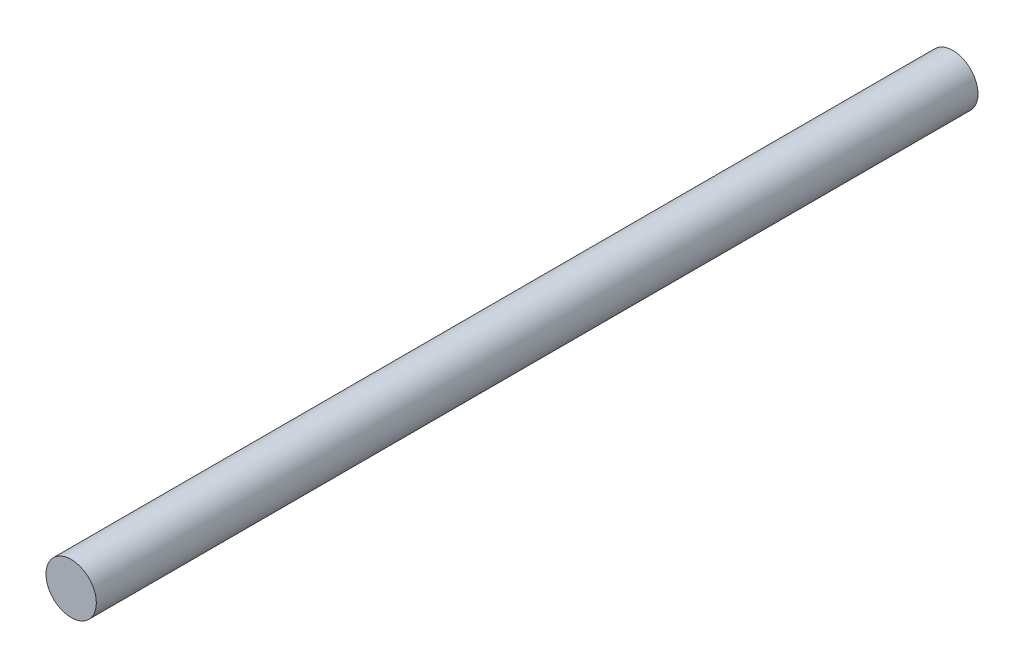
from build123d import *

# Parameters (mm, degrees)
SKETCH_1_R      = 2
EXTRUDE_1_DEPTH = 70


with BuildPart() as part:
    # 草图1 → 凸台-拉伸1 (new body)
    with BuildSketch(Plane.XY):
        Circle(SKETCH_1_R)
    extrude(amount=EXTRUDE_1_DEPTH)


solid = part.part
